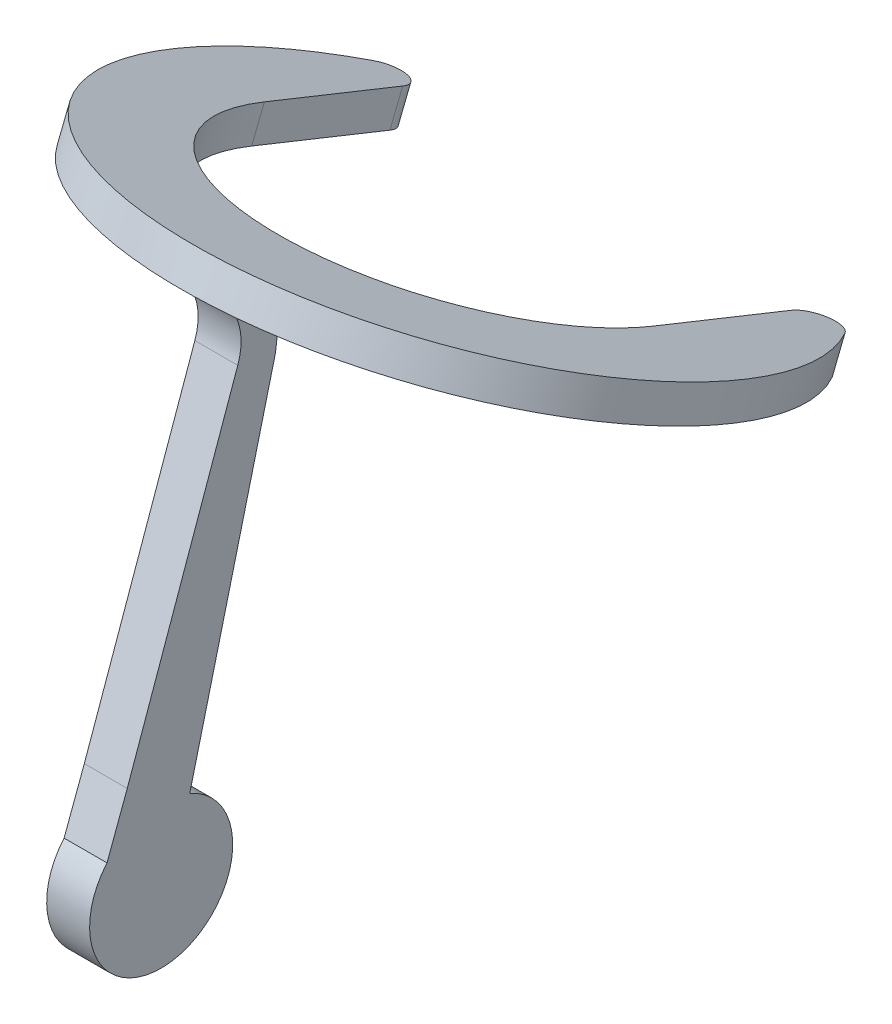
from build123d import *

# Parameters (mm, degrees)
SKETCH1_R           = 25
BOSS_EXTRUDE1_DEPTH = 7.5
BOSS_EXTRUDE2_DEPTH = 7.5
BOSS_EXTRUDE4_DEPTH = 12
FILLET1_R           = 20


with BuildPart() as part:
    # Sketch1 → Boss-Extrude1 (new, symmetric)
    with BuildSketch(Plane(origin=(0, 0, 0), x_dir=(0, 0, -1), z_dir=(1, 0, 0))):
        Circle(SKETCH1_R)
    extrude(amount=BOSS_EXTRUDE1_DEPTH, both=True)

    # Sketch2 → Boss-Extrude2 (add, symmetric)
    with BuildSketch(Plane(origin=(0, 0, 0), x_dir=(0, 0, -1), z_dir=(1, 0, 0))):
        Polygon((-25, 0), (-11.852856042, 35.333850942), (33.197452276, 162.153435325), (42.115400597, 158.580697497), (39.917408227, 141.125260536), (3.66577496, -1.999651309), align=None)
    extrude(amount=BOSS_EXTRUDE2_DEPTH, both=True)

    # Sketch4 → Boss-Extrude4 (add)
    with BuildSketch(Plane(origin=(0, 151.187639508, -60.569290091), x_dir=(1, 0, 0), z_dir=(0, 0.9282770434137098, -0.3718894065056191))):
        with BuildLine():
            Line((67.852060571, 102.029312181), (67.852060571, 49.967186724))
            ThreePointArc((67.852060571, 49.967186724), (0, -17.884873847), (-67.852060571, 49.967186724))
            Line((-67.852060571, 49.967186724), (-67.852060571, 102.029312181))
            ThreePointArc((-67.852060571, 102.029312181), (-73.482108128, 109.670210388), (-82.447891925, 106.556453525))
            ThreePointArc((-82.447891925, 106.556453525), (0, -50.032813276), (82.447891925, 106.556453525))
            ThreePointArc((82.447891925, 106.556453525), (73.482108128, 109.670210388), (67.852060571, 102.029312181))
        make_face()
    extrude(amount=BOSS_EXTRUDE4_DEPTH)

    # Fillet1
    fillet1_edges = [part.edges().sort_by_distance(p)[0] for p in [
        (0, 162.153435325, -33.197452276),
    ]]
    fillet(fillet1_edges, radius=FILLET1_R)


solid = part.part
